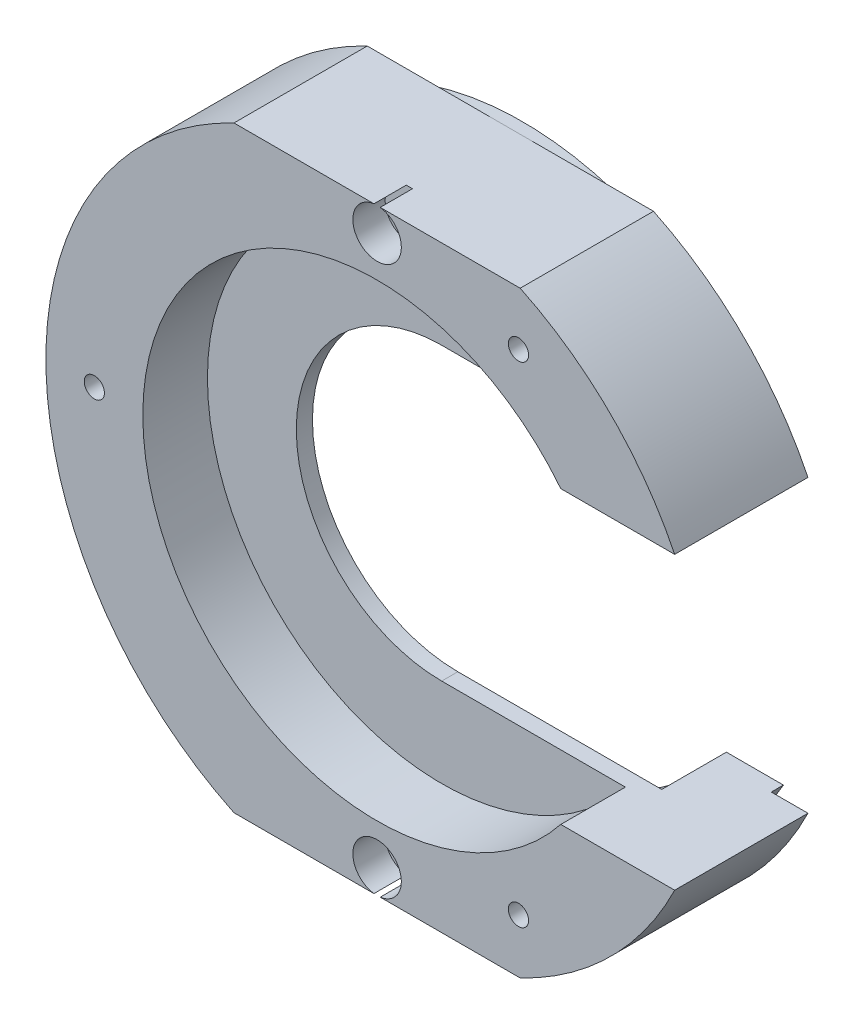
SolidWorks part; units mm, degrees
ref_plane "Front Plane" through (0, 0, 0) normal (0, 0, 1) x (1, 0, 0)
ref_plane "Top Plane" through (0, 0, 0) normal (0, 1, 0) x (1, 0, 0)
ref_plane "Right Plane" through (0, 0, 0) normal (1, 0, 0) x (0, 0, -1)
other "Configuration Table"
sketch "Sketch1" plane through (0, 0, 0) normal (0, 0, 1) x (1, 0, 0)
  circle A0 centre (0, 0) radius 41
  dimension "D1" = 82
extrude "Boss-Extrude1" add sketch "Sketch1" along normal blind 16.5
sketch "Sketch2" plane through (0, 0, 0) normal (0, 0, -1) x (-1, 0, 0)
  circle A0 centre (0, 0) radius 36.975
  dimension "D1" = 73.95
extrude "Boss-Extrude2" add sketch "Sketch2" along normal blind 1.5
sketch "Sketch4" plane through (0, 0, -1.5) normal (0, 0, -1) x (-1, 0, 0)
  line L0 (-25, 36.975) -> (25, 36.975) construction
  line L1 (0, 0) -> (11.911, 0) construction
  line L2 (-25, 36.975) -> (25, 36.975)
  line L3 (-25, 36.975) -> (-25, 43.815)
  line L4 (-25, 43.815) -> (25, 43.815)
  line L5 (25, 36.975) -> (25, 43.815)
  line L6 (25, -36.975) -> (25, -43.815)
  line L7 (-25, -43.815) -> (25, -43.815)
  line L8 (-25, -36.975) -> (25, -36.975)
  line L9 (-25, -36.975) -> (-25, -43.815)
  circle A1 centre (0, 0) radius 36.975 construction
  point P4 (0, 36.975)
  dimension "D1" = 6.84
  dimension "D2" = 50
extrude "Cut-Extrude1" cut sketch "Sketch4" against normal through all
sketch "Sketch5" plane through (0, 0, -1.5) normal (0, 0, -1) x (-1, 0, 0)
  circle A0 centre (0, 0) radius 31
  dimension "D1" = 62
extrude "Cut-Extrude3" cut sketch "Sketch5" against normal blind 8
sketch "Sketch6" plane through (0, 0, 16.5) normal (0, 0, 1) x (1, 0, 0)
  circle A0 centre (0, 0) radius 29
  dimension "D1" = 58
extrude "Cut-Extrude4" cut sketch "Sketch6" against normal blind 8
sketch "Sketch7" plane through (0, 0, 8.5) normal (0, 0, 1) x (1, 0, 0)
  line L0 (0, 18) -> (36.8375, 18)
  line L1 (0, -18) -> (36.8375, -18)
  arc A0 (0, 18) -> (0, -18) centre (0, 0) ccw
  arc A1 (17.7158, -36.975) -> (17.7158, 36.975) centre (0, 0) ccw construction
  arc A2 (36.8375, -18) -> (36.8375, 18) centre (0, 0) ccw
  dimension "D1" = 36
extrude "Cut-Extrude5" cut sketch "Sketch7" against normal through all both and the other way through all
sketch "Sketch8" plane through (0, 0, 16.5) normal (0, 0, 1) x (1, 0, 0)
  line L0 (0, 0) -> (-35, 0) construction
  line L1 (0, 34) -> (0, -34) construction
  circle A0 centre (0, 0) radius 35 construction
  circle A1 centre (0, 0) radius 34 construction
  dimension "D1" = 70
  dimension "D2" = 68
hole_wizard "CBORE for M3 Hex Head Bolt3" positions "3DSketch3" profile "Sketch12" counterbore size "M3" standard "GB" end condition through all
sketch3d "3DSketch3"
  point P0 (0, 34, 16.5)
  point P3 (0, 34, 16.5)
  point P5 (0, -34, 16.5)
  point P8 (0, -34, 16.5)
sketch "Sketch12" plane through (0, 34, 16.5) normal (1, 0, 0) x (0, -1, 0)
  line L0 (0, 0) -> (0, 18)
  line L1 (0, 18) -> (1.75, 18)
  line L3 (1.75, 18) -> (1.75, 4)
  line L4 (1.75, 4) -> (3, 4)
  line L5 (3, 4) -> (3, 0)
  line L7 (3, 0) -> (0, 0)
  line L11 (0, -6.35) -> (0, 107.95) construction
  dimension "通孔孔直径" = 3.5
  dimension "通孔孔深度" = 18
  dimension "柱形沉头孔直径" = 6
  dimension "柱形沉头孔深度" = 4
hole_wizard "M3 Tapped Hole1" positions "3DSketch4" profile "Sketch13" tap size "M3" standard "GB" end condition through all
sketch3d "3DSketch4"
  point P0 (-35, 0, 16.5)
  point P3 (-35, 0, 16.5)
sketch "Sketch13" plane through (-35, 0, 16.5) normal (1, 0, 0) x (0, -1, 0)
  line L0 (0, 0) -> (0, 18)
  line L1 (0, 18) -> (1.25, 18)
  line L2 (1.25, 18) -> (1.25, 0)
  line L5 (1.25, 0) -> (0, 0)
  line L11 (0, -6.35) -> (0, 107.95) construction
  dimension "通孔螺纹孔钻头直径" = 2.5
  dimension "通孔螺纹孔钻头深度" = 18
cosmetic thread "Cosmetic Thread2" parameters "D2"=3
pattern_circular "CirPattern1" count 3 over 360 about axis through (0, 0, 0) along (0, 0, 1) of "M3 Tapped Hole1"
